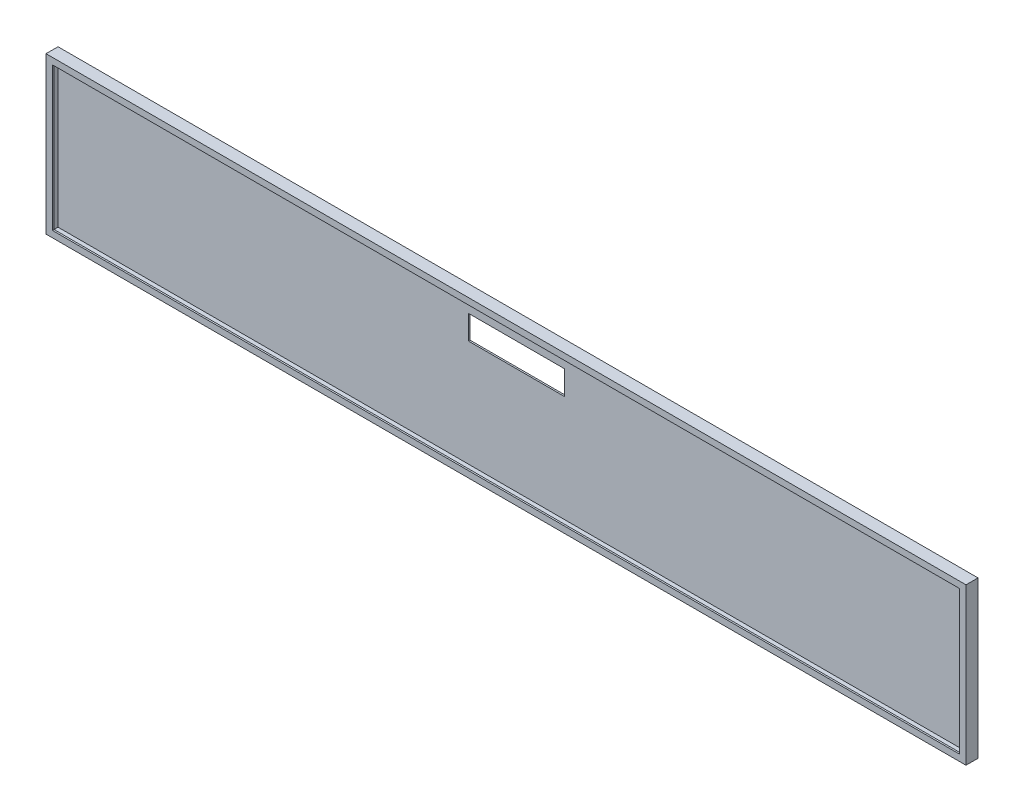
from build123d import *

# Parameters (mm, degrees)
SKETCH_1_W          = 1148
SKETCH_1_H          = 195
EXTRUDE_1_DEPTH     = 15
SHELL_1_T           = -2
SKETCH_2_W          = 1148
SKETCH_2_H          = 195
SKETCH_2_W_2        = 1132
SKETCH_2_H_2        = 179
EXTRUDE_2_DEPTH     = 2
SKETCH_3_W          = 120
SKETCH_3_H          = 30
CUT_EXTRUDE_1_DEPTH = 10


with BuildPart() as part:
    # 草图1 → 凸台-拉伸1 (new body)
    with BuildSketch(Plane.XY):
        with Locations((574, 97.5)):
            Rectangle(SKETCH_1_W, SKETCH_1_H)
    extrude(amount=EXTRUDE_1_DEPTH)

    # 抽壳1
    shell_1_openings = [part.faces().sort_by_distance(p)[0] for p in [
        (574, 97.5, 15),
    ]]
    offset(amount=SHELL_1_T, openings=shell_1_openings, kind=Kind.INTERSECTION)

    # 草图2 → 凸台-拉伸2 (add)
    with BuildSketch(Plane.XY.offset(15)):
        with Locations((574, 97.5)):
            Rectangle(SKETCH_2_W, SKETCH_2_H)
        with Locations((574, 97.5)):
            Rectangle(SKETCH_2_W_2, SKETCH_2_H_2, mode=Mode.SUBTRACT)
    extrude(amount=-EXTRUDE_2_DEPTH)

    # 草图3 → 切除-拉伸1 (cut)
    with BuildSketch(Plane(origin=(0, 0, 0), x_dir=(-1, 0, 0), z_dir=(0, 0, -1))):
        with Locations((-574, 150)):
            Rectangle(SKETCH_3_W, SKETCH_3_H)
    extrude(amount=-CUT_EXTRUDE_1_DEPTH, mode=Mode.SUBTRACT)


solid = part.part
